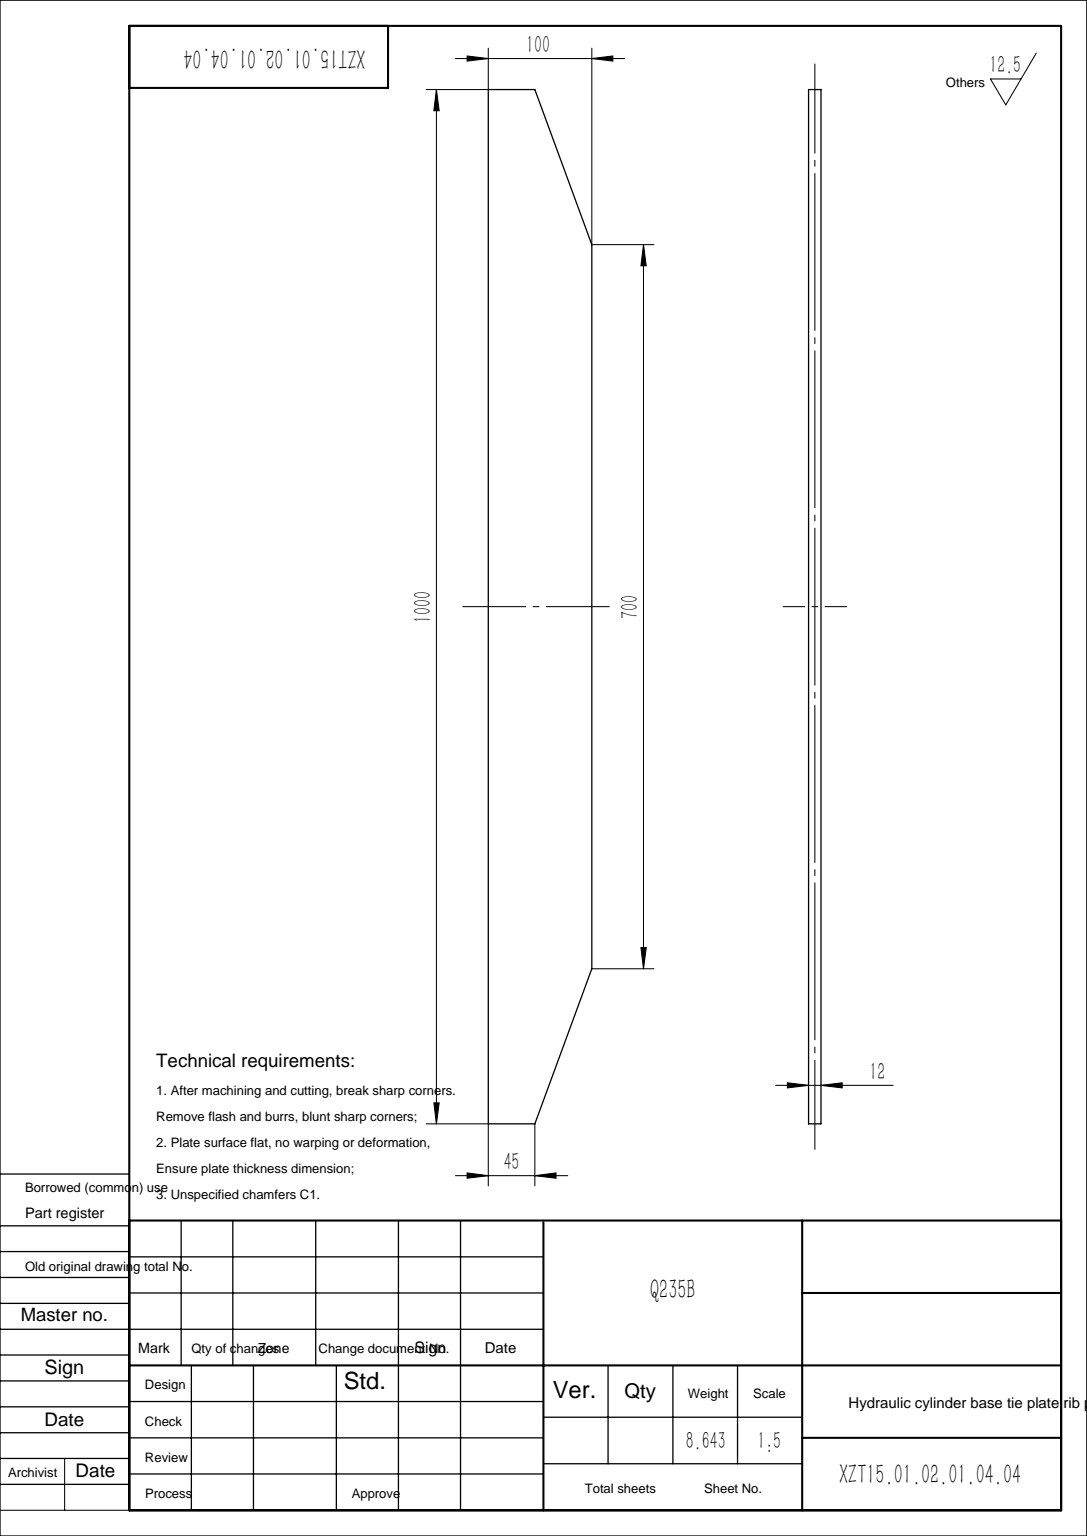
SolidWorks part; units mm, degrees
material "Q235B"
ref_plane "Front Plane" through (0, 0, 0) normal (0, 0, 1) x (1, 0, 0)
ref_plane "Top Plane" through (0, 0, 0) normal (0, 1, 0) x (1, 0, 0)
ref_plane "Right Plane" through (0, 0, 0) normal (1, 0, 0) x (0, 0, -1)
sketch "Sketch1" plane through (0, 0, 0) normal (0, 0, 1) x (1, 0, 0)
  line L0 (0, -500) -> (0, 500)
  line L1 (0, 500) -> (45, 500)
  line L2 (45, 500) -> (100, 350)
  line L3 (100, 350) -> (100, -350)
  line L4 (100, 0) -> (0, 0) construction
  line L5 (45, -500) -> (100, -350)
  line L6 (0, -500) -> (45, -500)
  dimension "D1" = 1000
  dimension "D2" = 700
  dimension "D3" = 100
  dimension "D4" = 45
extrude "Boss-Extrude1" add sketch "Sketch1" along normal mid plane 12
